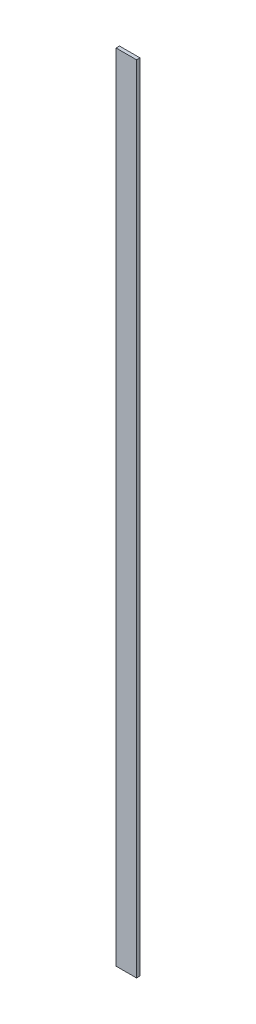
SolidWorks part; units mm, degrees
material "Q235"
ref_plane "Front Plane" through (0, 0, 0) normal (0, 0, 1) x (1, 0, 0)
ref_plane "Top Plane" through (0, 0, 0) normal (0, 1, 0) x (1, 0, 0)
ref_plane "Right Plane" through (0, 0, 0) normal (1, 0, 0) x (0, 0, -1)
sketch "Sketch1" plane through (0, 0, 0) normal (0, 0, 1) x (1, 0, 0)
  line L1 (0, 0) -> (60, 0)
  line L2 (0, 0) -> (0, 2330)
  line L3 (0, 2330) -> (60, 2330)
  line L4 (60, 0) -> (60, 2330)
  dimension "D1" = 60
  dimension "D2" = 2330
extrude "Boss-Extrude1" add sketch "Sketch1" along normal blind 10
